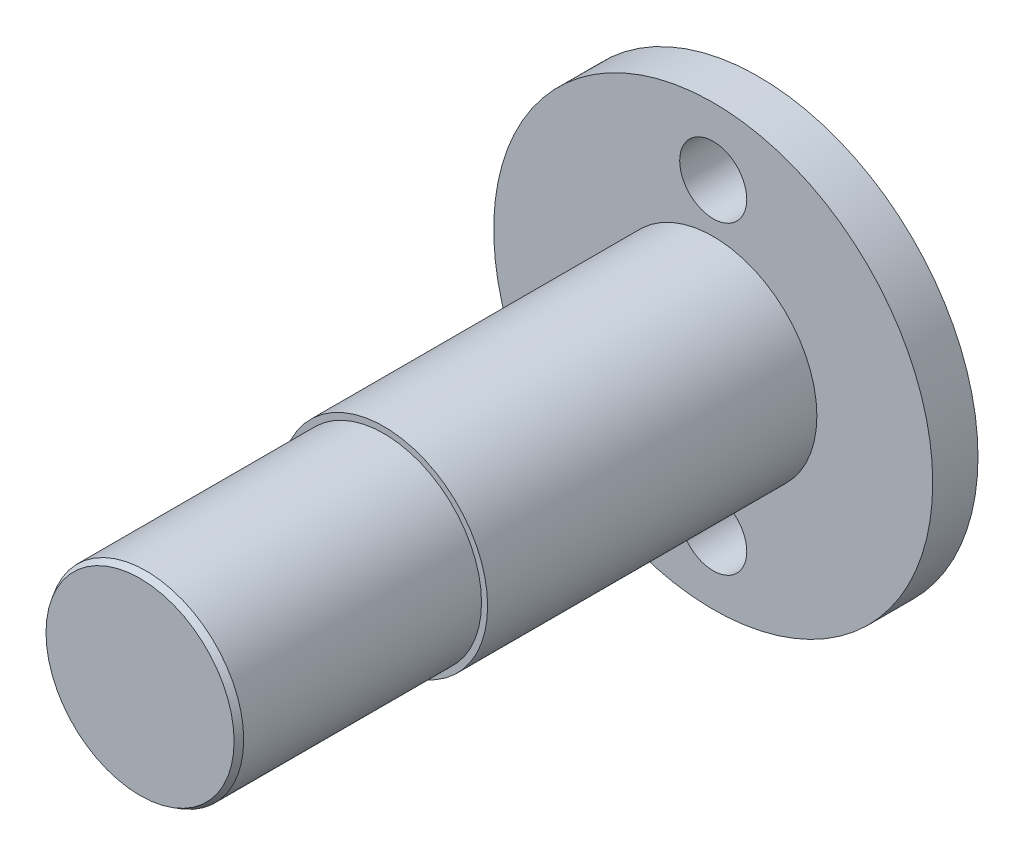
from build123d import *
from OCP.BRepFilletAPI import BRepFilletAPI_MakeChamfer

# Parameters (mm, degrees)
SKETCH1_R           = 18
BOSS_EXTRUDE1_DEPTH = 4
SKETCH2_R           = 8.5
BOSS_EXTRUDE2_DEPTH = 27
BOSS_EXTRUDE3_START = 27
SKETCH3_R           = 8
BOSS_EXTRUDE3_DEPTH = 20
CHAMFER1_SIZE       = 0.5
CHAMFER1_SIZE2      = 0.288675135
SKETCH4_R           = 2.75
CUT_EXTRUDE1_DEPTH  = 20


with BuildPart() as part:
    # Sketch1 → Boss-Extrude1 (new body)
    with BuildSketch(Plane.XY):
        Circle(SKETCH1_R)
    extrude(amount=BOSS_EXTRUDE1_DEPTH)

    # Sketch2 → Boss-Extrude2 (add)
    with BuildSketch(Plane.XY.offset(4)):
        Circle(SKETCH2_R)
    extrude(amount=BOSS_EXTRUDE2_DEPTH)

    # Sketch3 → Boss-Extrude3 (add)
    with BuildSketch(Plane.XY.offset(4).offset(BOSS_EXTRUDE3_START)):
        Circle(SKETCH3_R)
    extrude(amount=BOSS_EXTRUDE3_DEPTH)

    # Chamfer1: one chamfer whose edges measure the first distance from different faces: ONE call of the kernel's chamfer builder (chamfer() names one face for all edges)
    chamfer1_edges_1 = [part.edges().sort_by_distance(p)[0] for p in [
        (-8, 0, 51),
    ]]
    chamfer1_side_1 = [part.faces().sort_by_distance(p)[0] for p in [
        (-8, 0, 41),
    ]]
    chamfer1_edges_2 = [part.edges().sort_by_distance(p)[0] for p in [
        (-18, 0, 0),
    ]]
    chamfer1_side_2 = [part.faces().sort_by_distance(p)[0] for p in [
        (0, 0, 0),
    ]]
    chamfer1 = BRepFilletAPI_MakeChamfer(part.part.solid().wrapped)
    for e in chamfer1_edges_1:
        chamfer1.Add(CHAMFER1_SIZE, CHAMFER1_SIZE2, e.wrapped, chamfer1_side_1[0].wrapped)  # the first distance lies on this face
    for e in chamfer1_edges_2:
        chamfer1.Add(CHAMFER1_SIZE, CHAMFER1_SIZE2, e.wrapped, chamfer1_side_2[0].wrapped)  # the first distance lies on this face
    add(Compound.cast(chamfer1.Shape()), mode=Mode.REPLACE)

    # Sketch4 → Cut-Extrude1 (cut)
    with BuildSketch(Plane(origin=(0, 0, 0), x_dir=(-1, 0, 0), z_dir=(0, 0, -1))):
        with Locations((0, 12.5)):
            Circle(SKETCH4_R)
        with Locations((0, -12.5)):
            Circle(SKETCH4_R)
    extrude(amount=-CUT_EXTRUDE1_DEPTH, mode=Mode.SUBTRACT)


solid = part.part
